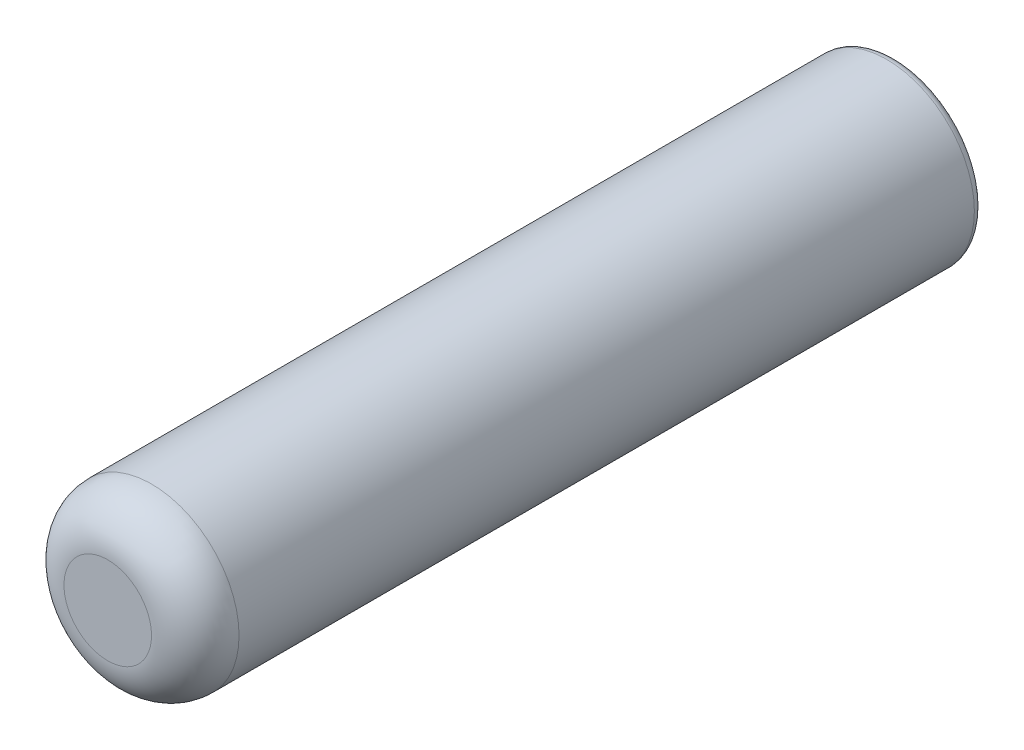
SolidWorks part; units mm, degrees
ref_plane "Front Plane" through (0, 0, 0) normal (0, 0, 1) x (1, 0, 0)
ref_plane "Top Plane" through (0, 0, 0) normal (0, 1, 0) x (1, 0, 0)
ref_plane "Right Plane" through (0, 0, 0) normal (1, 0, 0) x (0, 0, -1)
other "Configuration Table"
sketch "Sketch1" plane through (0, 0, 0) normal (0, 0, 1) x (1, 0, 0)
  circle A0 centre (0, 0) radius 1
  dimension "D1" = 2
extrude "Boss-Extrude1" add sketch "Sketch1" along normal blind 9
fillet "Fillet1" radius 0.5 1 edges at (1, 0, 9)
fillet "Fillet2" radius 0.1 1 edges at (1, 0, 0)
